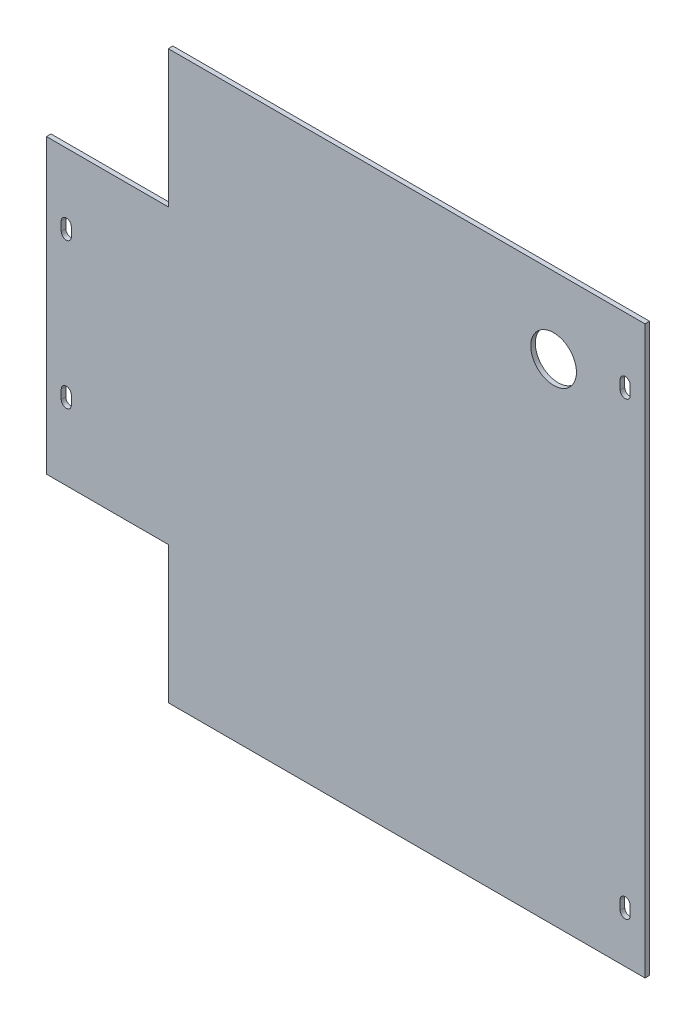
SolidWorks part; units mm, degrees
ref_plane "前视基准面" through (0, 0, 0) normal (0, 0, 1) x (1, 0, 0)
ref_plane "上视基准面" through (0, 0, 0) normal (0, 1, 0) x (1, 0, 0)
ref_plane "右视基准面" through (0, 0, 0) normal (1, 0, 0) x (0, 0, -1)
sketch "草图1" plane through (0, 0, 0) normal (0, 0, 1) x (1, 0, 0)
  line L1 (181.5, -186) -> (-181.5, -186)
  line L2 (181.5, -186) -> (181.5, 186)
  line L3 (181.5, 186) -> (-181.5, 186)
  line L4 (-181.5, -186) -> (-181.5, 186)
  line L5 (181.5, -186) -> (-181.5, 186) construction
  line L6 (181.5, 186) -> (-181.5, -186) construction
  point P0 (0, 0)
  dimension "D1" = 363
  dimension "D2" = 372
extrude "凸台-拉伸1" add sketch "草图1" along normal blind 3
sketch "草图2" plane through (0, 0, 3) normal (0, 0, 1) x (1, 0, 0)
  line L0 (181.5, -186) -> (181.5, 186) construction
  line L1 (181.5, 186) -> (-181.5, 186) construction
  circle A0 centre (121.5, 136) radius 15
  dimension "D1" = 30
  dimension "D2" = 60
  dimension "D3" = 50
extrude "切除-拉伸1" cut sketch "草图2" against normal blind 10
sketch "草图3" plane through (0, 0, 3) normal (0, 0, 1) x (1, 0, 0)
  line L1 (-131.5, -96) -> (-181.5, -96)
  line L2 (-131.5, -96) -> (-131.5, -186)
  line L3 (-131.5, -186) -> (-181.5, -186)
  line L4 (-181.5, -96) -> (-181.5, -186)
  line L5 (-131.5, -96) -> (-181.5, -186) construction
  line L6 (-131.5, -186) -> (-181.5, -96) construction
  line L7 (-131.5, 96) -> (-181.5, 96)
  line L8 (-131.5, 96) -> (-131.5, 186)
  line L9 (-131.5, 186) -> (-181.5, 186)
  line L10 (-181.5, 96) -> (-181.5, 186)
  line L11 (-131.5, 96) -> (-181.5, 186) construction
  line L12 (-131.5, 186) -> (-181.5, 96) construction
  point P0 (-156.5, -141)
  point P5 (-156.5, 141)
  dimension "D1" = 90
  dimension "D2" = 50
extrude "切除-拉伸2" cut sketch "草图3" against normal blind 10
sketch "草图4" plane through (-181.5, 0, 0) normal (-1, 0, 0) x (0, 0, 1)
  line L4 (0, 96) -> (0, -96)
  line L5 (0, -96) -> (3, -96)
  line L6 (3, -96) -> (3, 96)
  line L7 (3, 96) -> (0, 96)
  line L8 (0, 96) -> (0, -96)
  line L9 (0, -96) -> (3, -96)
  line L10 (3, -96) -> (3, 96)
  line L11 (3, 96) -> (0, 96)
  dimension "D1" = 0
extrude "凸台-拉伸2" add sketch "草图4" along normal blind 30
sketch "草图5" plane through (0, 0, 3) normal (0, 0, 1) x (1, 0, 0)
  line L8 (168.5, -155.5579) -> (168.5, -149.5579) construction
  line L9 (165.2, -155.5579) -> (165.2, -149.5579)
  line L10 (171.8, -155.5579) -> (171.8, -149.5579)
  line L11 (168.5, 140.2837) -> (168.5, 146.2837) construction
  line L12 (165.2, 140.2837) -> (165.2, 146.2837)
  line L13 (171.8, 140.2837) -> (171.8, 146.2837)
  line L14 (-198.5, 52.9197) -> (-198.5, 46.9197) construction
  line L15 (-195.2, 52.9197) -> (-195.2, 46.9197)
  line L16 (-198.5, -83) -> (-118.5, -83)
  line L17 (-118.5, -83) -> (-118.5, -173)
  line L18 (-118.5, -173) -> (168.5, -173)
  line L19 (168.5, -173) -> (168.5, 173)
  line L20 (168.5, 173) -> (-118.5, 173)
  line L21 (-118.5, 173) -> (-118.5, 83)
  line L22 (-118.5, 83) -> (-198.5, 83)
  line L23 (-198.5, 83) -> (-198.5, -83)
  line L27 (168.5, -173) -> (168.5, 173) construction
  line L31 (-198.5, 49.9197) -> (-198.5, -50.0803) construction
  line L32 (-201.8, 52.9197) -> (-201.8, 46.9197)
  line L33 (-198.5, -48.7149) -> (-198.5, -42.7149) construction
  line L34 (-201.8, -48.7149) -> (-201.8, -42.7149)
  line L35 (-195.2, -48.7149) -> (-195.2, -42.7149)
  arc A0 (165.2, -155.5579) -> (171.8, -155.5579) centre (168.5, -155.5579) ccw
  arc A1 (171.8, -149.5579) -> (165.2, -149.5579) centre (168.5, -149.5579) ccw
  arc A2 (165.2, 140.2837) -> (171.8, 140.2837) centre (168.5, 140.2837) ccw
  arc A3 (171.8, 146.2837) -> (165.2, 146.2837) centre (168.5, 146.2837) ccw
  arc A4 (-195.2, 52.9197) -> (-201.8, 52.9197) centre (-198.5, 52.9197) ccw
  arc A5 (-201.8, 46.9197) -> (-195.2, 46.9197) centre (-198.5, 46.9197) ccw
  arc A6 (-201.8, -48.7149) -> (-195.2, -48.7149) centre (-198.5, -48.7149) ccw
  arc A7 (-195.2, -42.7149) -> (-201.8, -42.7149) centre (-198.5, -42.7149) ccw
  point P2 (168.5, -152.5579)
  point P9 (168.5, 143.2837)
  dimension "D2" = 3.3
  dimension "D3" = 6
  dimension "D4" = 100
  dimension "D1" = 13
extrude "切除-拉伸3" cut sketch "草图5" against normal blind 10
